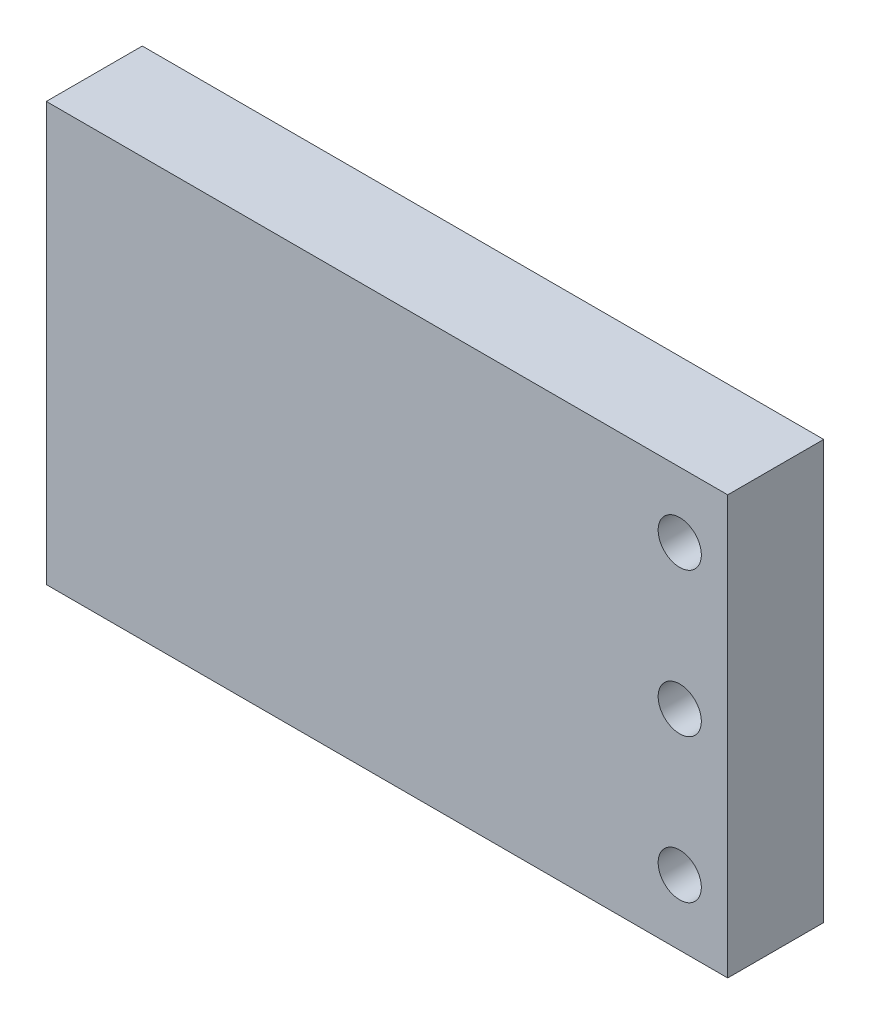
from build123d import *

# Parameters (mm, degrees)
SKETCH_1_W                   = 71
SKETCH_1_H                   = 10
EXTRUDE_1_DEPTH              = 43.6
HOLE_WIZARD_M4_1_D           = 4.5
HOLE_WIZARD_M4_1_CBORE_D     = 8
HOLE_WIZARD_M4_1_CBORE_DEPTH = 4.6
HOLE_WIZARD_M4_1_2_D         = 3.3
HOLE_WIZARD_M4_1_2_DEPTH     = 10.1
HOLE_WIZARD_M4_1_2_TIP       = 0.991420021


with BuildPart() as part:
    # 草图1 → 凸台-拉伸1 (new body)
    with BuildSketch(Plane(origin=(0, 0, 0), x_dir=(1, 0, 0), z_dir=(0, 1, 0))):
        with Locations((35.5, 5)):
            Rectangle(SKETCH_1_W, SKETCH_1_H)
    extrude(amount=EXTRUDE_1_DEPTH)

    # Hole Wizard M4 _1 (through all)
    with Locations(Plane(origin=(0, 0, -10), x_dir=(-1, 0, 0), z_dir=(0, 0, -1))):
        with Locations((-66, 36.8), (-66, 21.783451384), (-66, 6.8)):
            CounterBoreHole(HOLE_WIZARD_M4_1_D / 2, HOLE_WIZARD_M4_1_CBORE_D / 2, HOLE_WIZARD_M4_1_CBORE_DEPTH)

    # Hole Wizard M4 _1 2
    with Locations(Plane.ZY):
        with Locations((-5, 37.8), (-5, 21.8), (-5, 5.8)):
            Hole(HOLE_WIZARD_M4_1_2_D / 2, depth=HOLE_WIZARD_M4_1_2_DEPTH)
            with Locations((0, 0, -(HOLE_WIZARD_M4_1_2_DEPTH + HOLE_WIZARD_M4_1_2_TIP / 2))):  # 118° drill point
                Cone(0, HOLE_WIZARD_M4_1_2_D / 2, HOLE_WIZARD_M4_1_2_TIP, mode=Mode.SUBTRACT)


solid = part.part
